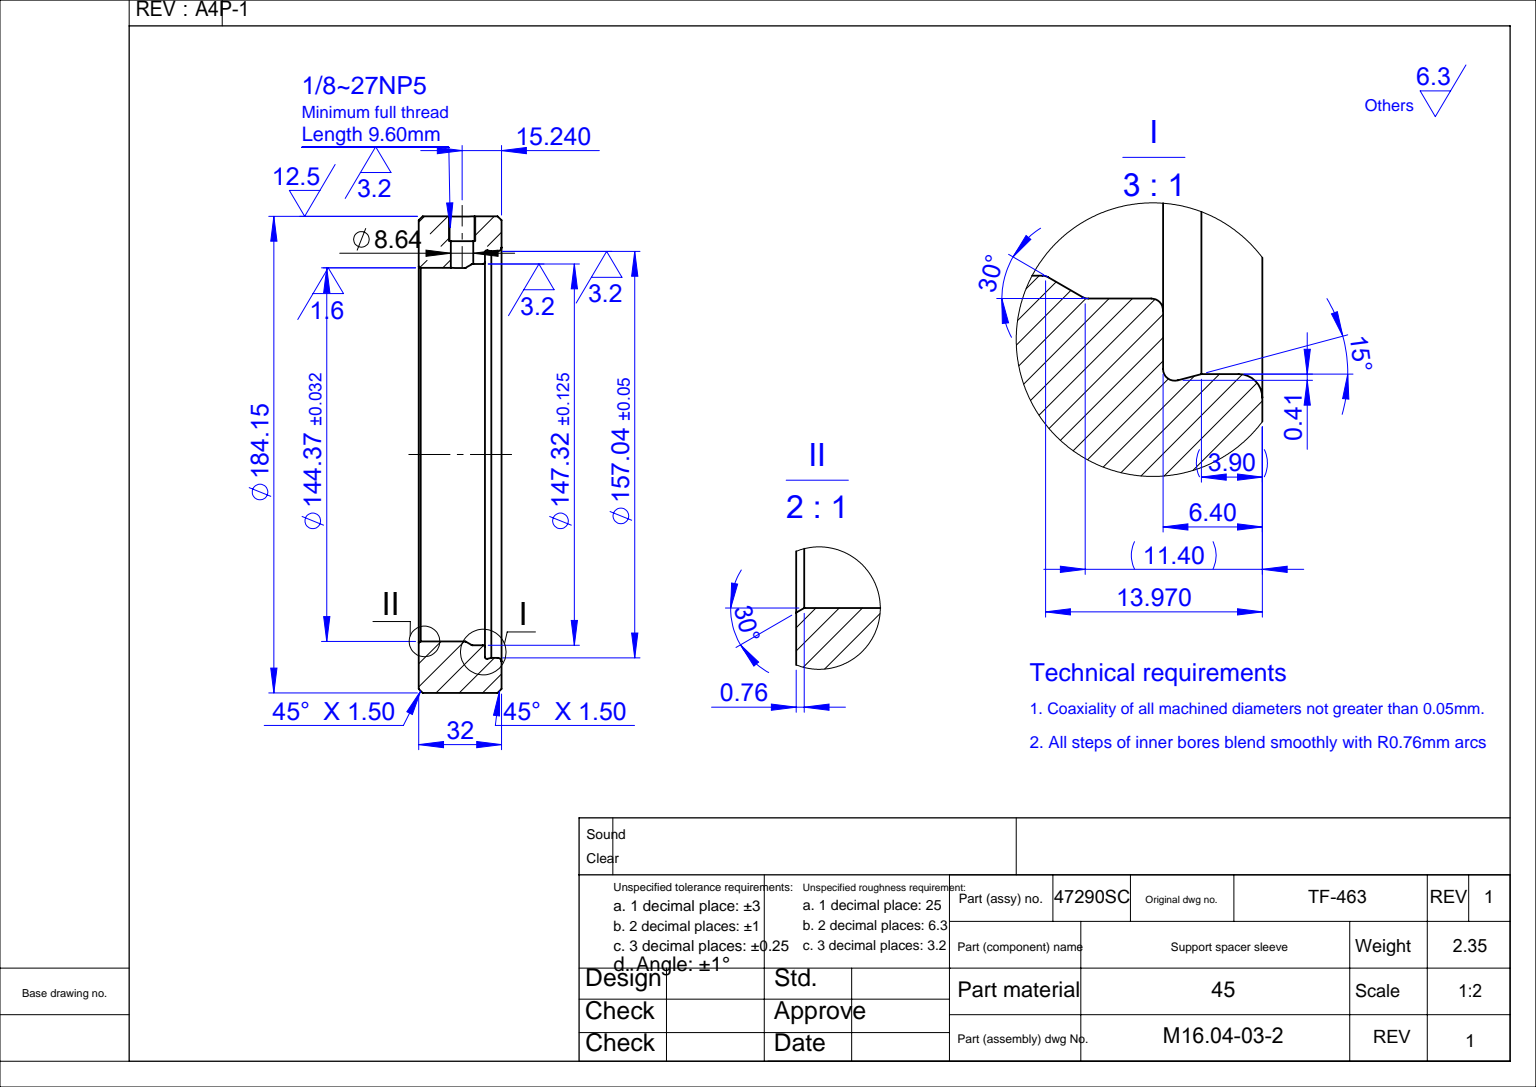
from build123d import *
from build123d.topology import SkipClean

# Parameters (mm, degrees)
CHAMFER2_SIZE                      = 0.762
CHAMFER2_SIZE2                     = 0.439940905
CHAMFER3_SIZE                      = 1.524
F_1_8_NPT_TAPPED_HOLE1_D           = 8.636
F_1_8_NPT_TAPPED_HOLE1_DEPTH       = 19.431
F_1_8_NPT_TAPPED_HOLE1_CBORE_D     = 9.6527874
F_1_8_NPT_TAPPED_HOLE1_CBORE_DEPTH = 9.652
F_1_8_NPT_TAPPED_HOLE1_TIP         = 2.594516153
SKETCH4_R                          = 4.318
CUT_EXTRUDE1_DEPTH                 = 82.423


with BuildPart() as part:
    # Sketch1 → Revolve1 (revolve)
    with BuildSketch(Plane.XY, mode=Mode.PRIVATE) as revolve1_sk:
        with BuildLine():
            Line((0, 92.075), (32, 92.075))
            Line((32, 92.075), (32, 80.044))
            ThreePointArc((32, 80.044), (31.553630735, 78.966369265), (30.476, 78.52))
            Line((30.476, 78.52), (28.075925561, 78.52))
            Line((28.075925561, 78.52), (26.559220112, 78.9264))
            ThreePointArc((26.559220112, 78.9264), (25.898123791, 78.794899766), (25.6, 78.19036452))
            Line((25.6, 78.19036452), (25.6, 74.422))
            ThreePointArc((25.6, 74.422), (25.376815367, 73.883184633), (24.838, 73.66))
            Line((24.838, 73.66), (20.785834534, 73.66))
            ThreePointArc((20.785834534, 73.66), (20.588614422, 73.63403548), (20.404834534, 73.557911358))
            Line((20.404834534, 73.557911358), (18.206822715, 72.288888642))
            ThreePointArc((18.206822715, 72.288888642), (18.023042828, 72.21276452), (17.825822715, 72.1868))
            Line((17.825822715, 72.1868), (0, 72.1868))
            Line((0, 72.1868), (0, 92.075))
        make_face()
    revolve(revolve1_sk.sketch.rotate(Axis((-48.080119454, 0, 0), (1, 0, 0)), 90), axis=Axis((-48.080119454, 0, 0), (1, 0, 0)))

    # Chamfer2
    chamfer2_edges = [part.edges().sort_by_distance(p)[0] for p in [
        (0, 0, -72.1868),
    ]]
    chamfer2_side = [part.faces().sort_by_distance(p)[0] for p in [
        (8.912911358, 0, -72.1868),
    ]]
    chamfer(chamfer2_edges, length=CHAMFER2_SIZE, length2=CHAMFER2_SIZE2, reference=chamfer2_side[0])

    # Chamfer3
    chamfer3_edges = [part.edges().sort_by_distance(p)[0] for p in [
        (32, 0, -92.075),
        (0, 0, -92.075),
    ]]
    chamfer(chamfer3_edges, length=CHAMFER3_SIZE)

    # 1/8 NPT Tapped Hole1
    with Locations(Plane(origin=(16.76, 92.075, 0), x_dir=(0, 0, 1), z_dir=(0, 1, 0))):
        with Locations((0, 0)):
            CounterBoreHole(F_1_8_NPT_TAPPED_HOLE1_D / 2, F_1_8_NPT_TAPPED_HOLE1_CBORE_D / 2, F_1_8_NPT_TAPPED_HOLE1_CBORE_DEPTH, depth=F_1_8_NPT_TAPPED_HOLE1_DEPTH)
            with Locations((0, 0, -(F_1_8_NPT_TAPPED_HOLE1_DEPTH + F_1_8_NPT_TAPPED_HOLE1_TIP / 2))):  # 118° drill point
                Cone(0, F_1_8_NPT_TAPPED_HOLE1_D / 2, F_1_8_NPT_TAPPED_HOLE1_TIP, mode=Mode.SUBTRACT)

    # Sketch4 → Cut-Extrude1 (cut)
    with SkipClean():  # the faces are left unmerged after this step: merging them gives an invalid solid
        with BuildSketch(Plane(origin=(0, 0, 0), x_dir=(1, 0, 0), z_dir=(0, 1, 0))):
            with Locations(Location((16.76, 0, 0), (0, 0, 270))):
                Circle(SKETCH4_R)
        extrude(amount=CUT_EXTRUDE1_DEPTH, mode=Mode.SUBTRACT)


solid = part.part
